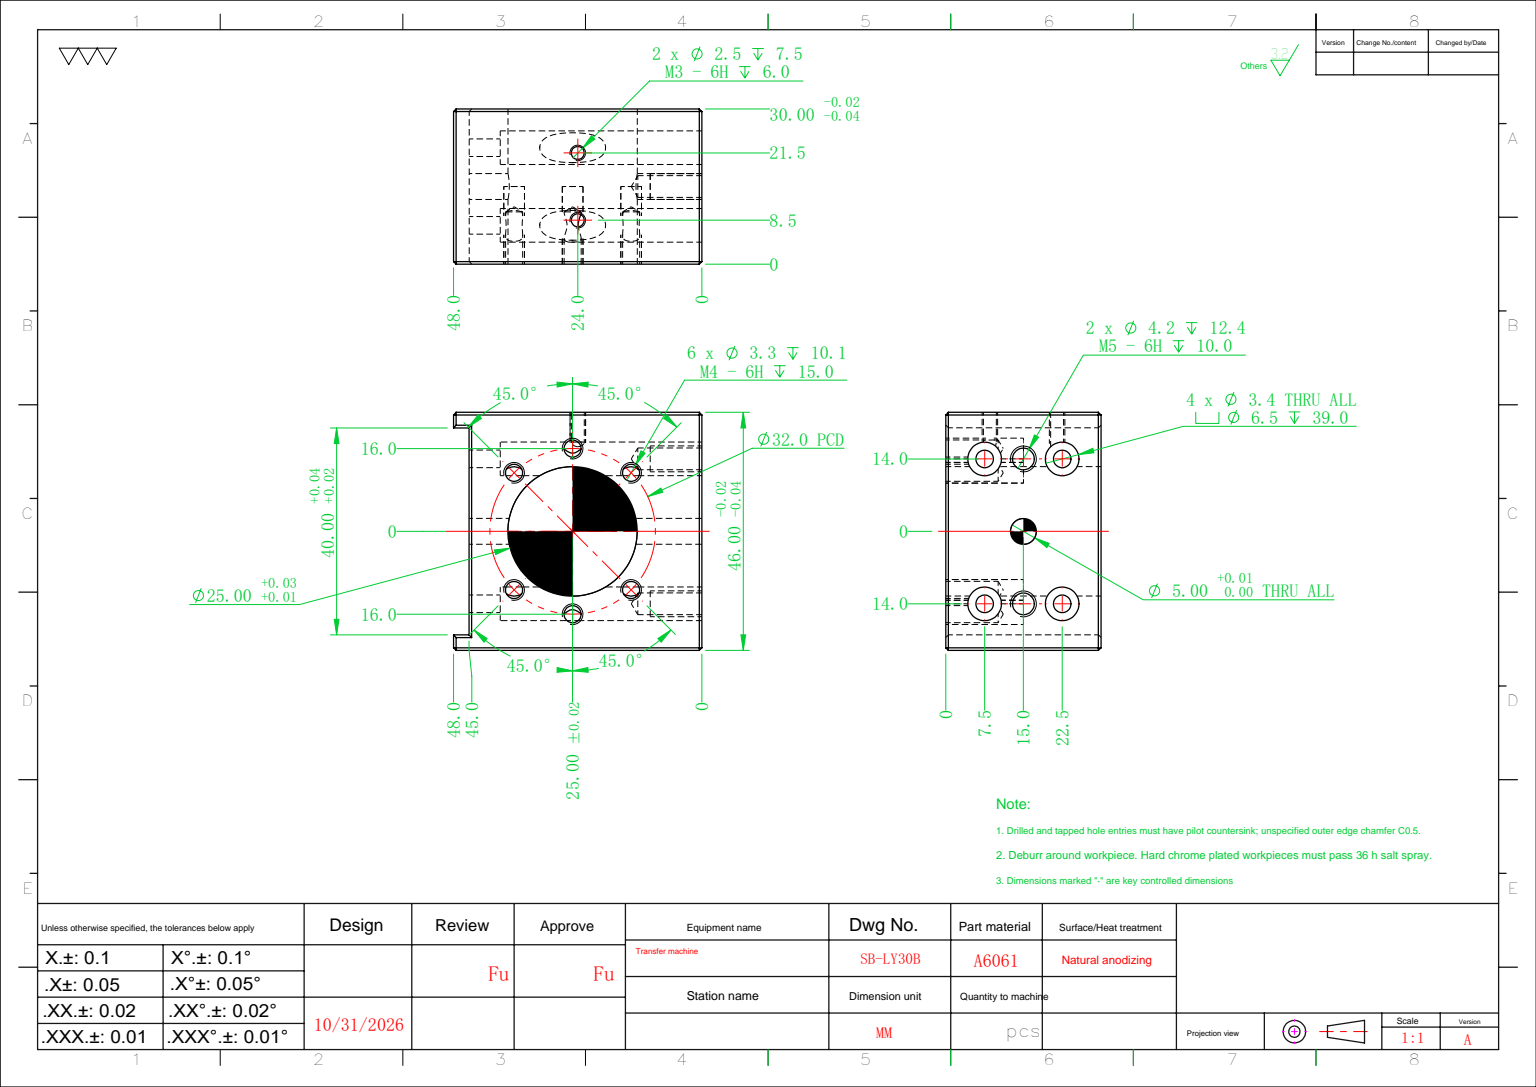
SolidWorks part; units mm, degrees
ref_plane "前视基准面" through (0, 0, 0) normal (0, 0, 1) x (1, 0, 0)
ref_plane "上视基准面" through (0, 0, 0) normal (0, 1, 0) x (1, 0, 0)
ref_plane "右视基准面" through (0, 0, 0) normal (1, 0, 0) x (0, 0, -1)
sketch "草图1" plane through (0, 0, 0) normal (0, 0, 1) x (1, 0, 0)
  line L1 (-23, -24) -> (23, -24)
  line L2 (-23, -24) -> (-23, 24)
  line L3 (-23, 24) -> (23, 24)
  line L4 (23, -24) -> (23, 24)
  line L5 (-23, -24) -> (23, 24) construction
  line L6 (-23, 24) -> (23, -24) construction
  point P0 (0, 0)
  dimension "D1" = 46
  dimension "D2" = 48
extrude "凸台-拉伸1" add sketch "草图1" along normal blind 30
sketch "草图2" plane through (0, 0, 30) normal (0, 0, 1) x (1, 0, 0)
  line L0 (-23, -24) -> (23, -24) construction
  line L1 (-20, -24) -> (20, -24)
  line L2 (-20, -24) -> (-20, -21)
  line L3 (-20, -21) -> (20, -21)
  line L4 (20, -24) -> (20, -21)
  line L5 (0, 0) -> (0, -29.6007) construction
  dimension "D1" = 40
  dimension "D2" = 3
extrude "切除-拉伸1" cut sketch "草图2" against normal through all
hole_wizard "M3 六角凹头螺钉的柱形沉头孔1" positions "草图3" profile "草图4" counterbore size "M3" standard "ISO" end condition through all
sketch "草图3" plane through (0, 24, 0) normal (0, 1, 0) x (1, 0, 0)
  line L0 (0, 0) -> (0, -30) construction
  line L1 (23, -30) -> (-23, -30) construction
  line L3 (-23, -15) -> (23, -15) construction
  line L4 (-23, -30) -> (-23, 0) construction
  line L5 (23, -30) -> (23, 0) construction
  point P0 (-14, -7.5)
  point P16 (14, -7.5)
  point P17 (14, -22.5)
  point P18 (-14, -22.5)
  dimension "D1" = 28
  dimension "D2" = 15
sketch "草图4" plane through (-14, 24, 7.5) normal (1, 0, 0) x (0, 0, 1)
  line L0 (0, 0) -> (0, 48)
  line L1 (0, 48) -> (1.7, 48)
  line L3 (1.7, 48) -> (1.7, 39)
  line L4 (1.7, 39) -> (3.25, 39)
  line L5 (3.25, 39) -> (3.25, 0)
  line L7 (3.25, 0) -> (0, 0)
  line L11 (0, -6.35) -> (0, 107.95) construction
  dimension "通孔孔直径" = 3.4
  dimension "通孔孔深度" = 48
  dimension "柱形沉头孔直径" = 6.5
  dimension "柱形沉头孔深度" = 39
sketch "草图5" plane through (0, 0, 30) normal (0, 0, 1) x (1, 0, 0)
  line L0 (0, 24) -> (0, -21) construction
  line L1 (23, 24) -> (-23, 24) construction
  line L2 (20, -21) -> (-20, -21) construction
  line L4 (-23, -24) -> (-20, -24) construction
  circle A0 centre (0, -1) radius 12.5
  dimension "D1" = 25
  dimension "D2" = 23
extrude "切除-拉伸2" cut sketch "草图5" against normal through all
hole_wizard "大小mm 暗销孔1" positions "草图13" profile "草图14" hole size "Ø5.0" standard "ISO" end condition through all
sketch "草图13" plane through (0, 24, 0) normal (0, 1, 0) x (1, 0, 0)
  line L0 (0, 0) -> (0, -30) construction
  line L1 (23, -30) -> (-23, -30) construction
  point P0 (0, -15)
sketch "草图14" plane through (0, 24, 15) normal (1, 0, 0) x (0, 0, 1)
  line L0 (0, 0) -> (0, 48)
  line L1 (0, 48) -> (2.5, 48)
  line L2 (2.5, 48) -> (2.5, 0)
  line L5 (2.5, 0) -> (0, 0)
  line L11 (0, -6.35) -> (0, 107.95) construction
  dimension "通孔孔直径" = 5
  dimension "通孔孔深度" = 48
chamfer "倒角1" distance 0.5 angle 45 20 edges at (-23, 24, 15) (-23, -24, 15) (-23, 0, 30) (0, 24, 30) (-21.5, -24, 30) (-20, -22.5, 30) (20, -22.5, 30) (21.5, -24, 30) (23, -24, 15) (23, 0, 30) (23, 24, 15) (20, -22.5, 0) (21.5, -24, 0) (0, 24, 0) (-23, 0, 0) (-21.5, -24, 0) (-20, -22.5, 0) (0, -21, 30) (0, -21, 0) (23, 0, 0)
hole_wizard "M5 螺纹孔1" positions "草图15" profile "草图16" tap size "M5" standard "ISO"
sketch "草图15" plane through (0, 24, 0) normal (0, 1, 0) x (1, 0, 0)
  line L0 (-14, -22.5) -> (-14, -7.5) construction
  line L2 (14, -22.5) -> (14, -7.5) construction
  point P0 (-14, -15)
  point P2 (14, -15)
sketch "草图16" plane through (-14, 24, 15) normal (1, 0, 0) x (0, 0, 1)
  line L0 (0, 0) -> (0, 13.6618)
  line L1 (0, 13.6618) -> (2.1, 12.4)
  line L2 (2.1, 12.4) -> (2.1, 0)
  line L5 (2.1, 0) -> (0, 0)
  line L10 (0, 13.6618) -> (-2.1, 12.4) construction
  line L11 (0, -6.35) -> (0, 107.95) construction
  dimension "螺纹孔钻头直径" = 4.2
  dimension "螺纹孔钻头深度" = 12.4
  dimension "导头角度" = 118
cosmetic thread "孔螺蚊线1" parameters "D1"=10, "D2"=5
cosmetic thread "孔螺蚊线2" parameters "D1"=10, "D2"=5
hole_wizard "M3 螺纹孔2" positions "草图19" profile "草图20" tap size "M3" standard "ISO"
sketch "草图19" plane through (23, 0, 0) normal (1, 0, 0) x (0, 0, -1)
  line L3 (-0.5, -24) -> (-29.5, -24) construction
  line L4 (-15, 23.5) -> (-15, -18.1516) construction
  line L5 (-0.5, 23.5) -> (-29.5, 23.5) construction
  point P0 (-21.5, 0)
  point P2 (-8.5, 0)
  dimension "D1" = 13
  dimension "D2" = 24
sketch "草图20" plane through (23, 0, 21.5) normal (0, 1, 0) x (0, 0, -1)
  line L0 (0, 0) -> (0, 8.2511)
  line L1 (0, 8.2511) -> (1.25, 7.5)
  line L2 (1.25, 7.5) -> (1.25, 0)
  line L5 (1.25, 0) -> (0, 0)
  line L10 (0, 8.2511) -> (-1.25, 7.5) construction
  line L11 (0, -6.35) -> (0, 107.95) construction
  dimension "螺纹孔钻头直径" = 2.5
  dimension "螺纹孔钻头深度" = 7.5
  dimension "导头角度" = 118
cosmetic thread "孔螺蚊线7" parameters "D1"=6, "D2"=3
cosmetic thread "孔螺蚊线8" parameters "D1"=6, "D2"=3
hole_wizard "M4 螺纹孔1" positions "草图21" profile "草图22" tap size "M4" standard "ISO"
sketch "草图21" plane through (0, 0, 0) normal (0, 0, -1) x (-1, 0, 0)
  line L0 (-16, -1) -> (0, -1) construction
  line L1 (0, -1) -> (0, 8.3017) construction
  line L3 (0, -1) -> (-11.3137, 10.3137) construction
  point P0 (-16, -1)
  point P13 (-11.3137, 10.3137)
  point P19 (11.3137, 10.3137)
  point P20 (16, -1)
  point P21 (11.3137, -12.3137)
  point P22 (-11.3137, -12.3137)
  dimension "D1" = 32
  dimension "D2" = 45
sketch "草图22" plane through (16, -1, 0) normal (1, 0, 0) x (0, 1, 0)
  line L0 (0, 0) -> (0, 11.0914)
  line L1 (0, 11.0914) -> (1.65, 10.1)
  line L2 (1.65, 10.1) -> (1.65, 0)
  line L5 (1.65, 0) -> (0, 0)
  line L10 (0, 11.0914) -> (-1.65, 10.1) construction
  line L11 (0, -6.35) -> (0, 107.95) construction
  dimension "螺纹孔钻头直径" = 3.3
  dimension "螺纹孔钻头深度" = 10.1
  dimension "导头角度" = 118
cosmetic thread "孔螺蚊线9" parameters "D1"=15, "D2"=4
cosmetic thread "孔螺蚊线10" parameters "D1"=15, "D2"=4
cosmetic thread "孔螺蚊线11" parameters "D1"=15, "D2"=4
cosmetic thread "孔螺蚊线12" parameters "D1"=15, "D2"=4
cosmetic thread "孔螺蚊线13" parameters "D1"=15, "D2"=4
cosmetic thread "孔螺蚊线14" parameters "D1"=15, "D2"=4
